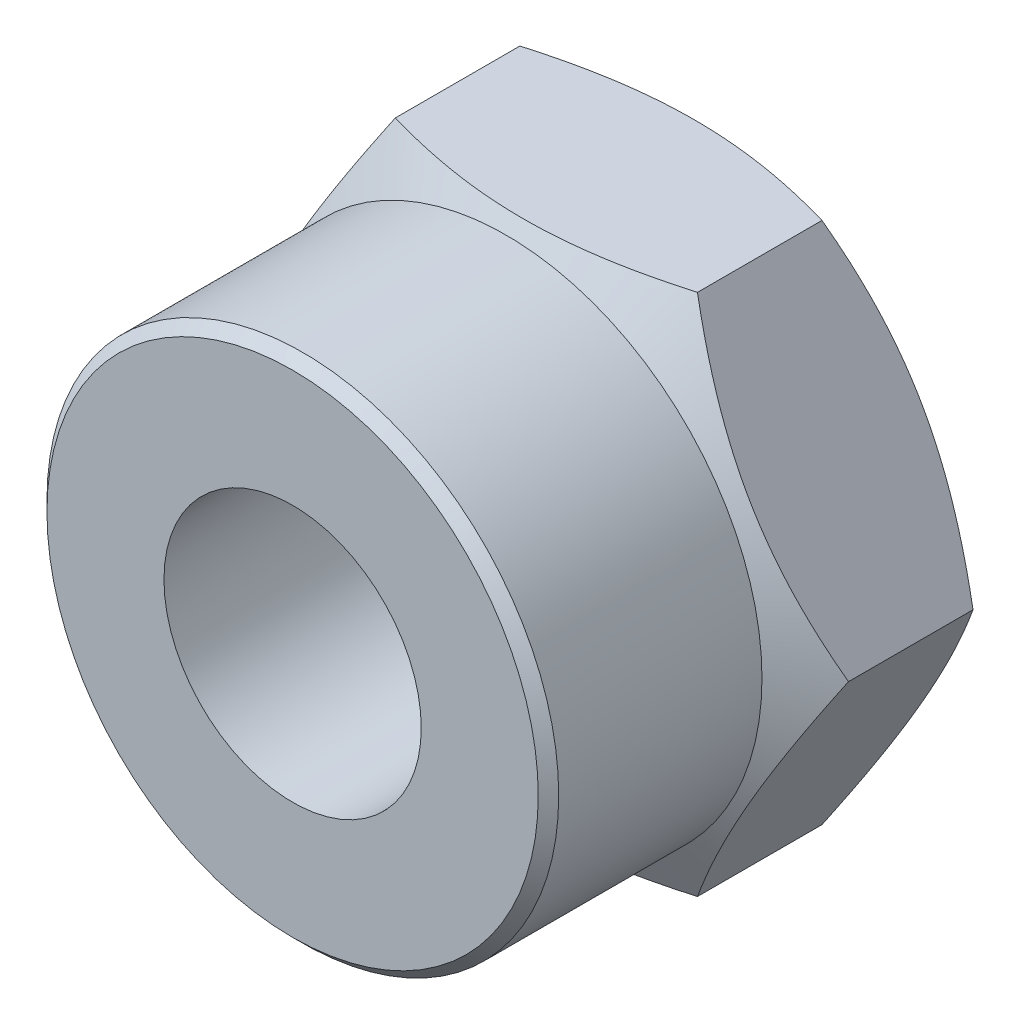
SolidWorks part; units mm, degrees
ref_plane "Front" through (0, 0, 0) normal (0, 0, 1) x (1, 0, 0)
ref_plane "Top" through (0, 0, 0) normal (0, 1, 0) x (1, 0, 0)
ref_plane "Right" through (0, 0, 0) normal (1, 0, 0) x (0, 0, -1)
sketch "Sketch1" plane through (0, 0, 0) normal (0, 0, 1) x (1, 0, 0)
  line L1 (2.8868, -5) -> (5.7735, 0)
  line L2 (5.7735, 0) -> (2.8868, 5)
  line L3 (2.8868, 5) -> (-2.8868, 5)
  line L4 (-2.8868, 5) -> (-5.7735, 0)
  line L5 (-5.7735, 0) -> (-2.8868, -5)
  line L6 (-2.8868, -5) -> (2.8868, -5)
  circle A0 centre (0, 0) radius 5 construction
  circle A1 centre (0, 0) radius 2.4585
extrude "BaseNut" add sketch "Sketch1" against normal blind 3.92
cosmetic thread "ThreadCosmetic1" [suppressed] parameters "m"=4.9, "D2"=6
sketch "Sketch3" plane through (0, 0, 0) normal (0, 1, 0) x (1, 0, 0)
  line L0 (0, 16.3108) -> (0, -16.1137) construction
  line L2 (-2.0696, 1.96) -> (33.5085, 1.96) construction
  line L3 (4.44, 3.92) -> (5.7735, 3.92)
  line L5 (5.7735, 3.92) -> (5.7735, 3.1501)
  line L7 (5.7735, 3.1501) -> (4.44, 3.92)
  line L8 (5.7735, 0.7699) -> (4.44, 0)
  line L9 (5.7735, 0) -> (5.7735, 0.7699)
  line L10 (4.44, 0) -> (5.7735, 0)
  dimension "D1" = 30
  dimension "dw" = 8.88
revolve "Double-Chamfer" cut sketch "Sketch3" angle 360 about L0
sketch "Sketch2" plane through (20.0871, -4.2815, 0) normal (0, 0, 1) x (1, 0, 0)
  circle A1 centre (-20.0871, 4.2815) radius 2.4585 construction
  circle A2 centre (-20.0871, 4.2815) radius 4.89
  circle A3 centre (-20.0871, 4.2815) radius 2.4585
extrude "Extrude1" add sketch "Sketch2" along normal offset from surface (4.08 mm away) 8 up to face at (2.4585, 0, -3.92)
sketch "Sketch5" plane through (0, 0, 0) normal (0, 1, 0) x (1, 0, 0)
  line L0 (0, 16.8008) -> (0, -2.8116) construction
  line L2 (2.4585, 3.92) -> (3.375, 3.92)
  line L5 (3.375, 3.92) -> (2.4585, 3.0035)
  line L7 (2.4585, 3.0035) -> (2.4585, 3.92)
  dimension "D1" = 45
  dimension "da" = 6.75
revolve "EndChamfer" cut sketch "Sketch5" angle 360 about L0
chamfer "Chamfer1" distance 0.1956 angle 45 1 edges at (4.89, 0, 4.08)
sketch "Sketch6" plane through (0, 0, 0) normal (0, 1, 0) x (1, 0, 0)
  line L0 (0, 30.0005) -> (0, -32.7386) construction
  line L1 (1.917, 3.2743) -> (2.4585, 3.2743)
  line L2 (2.4585, 3.2743) -> (2.9275, 3.0035)
  line L3 (2.9275, 3.0035) -> (2.4585, 2.7328)
  line L4 (2.4585, 2.7328) -> (1.917, 2.7328)
  line L5 (1.917, 2.7328) -> (1.917, 3.2743)
  line L6 (-2.4585, 3.0035) -> (2.4585, 3.0035) construction
revolve "Cut-Revolve10" [suppressed] cut sketch "Sketch6" angle 360 about L0
pattern_linear "LPattern10" [suppressed] count 6 spacing 0.6498 along (0, 0, 1)
equation "\"D1@Chamfer1\" = \"s1@Sketch2\" / 50"
equation "\"D2@Sketch6\" = \"xd@Sketch1\""
equation "\"D1@Sketch6\" = (  \"D2@ThreadCosmetic1\" - \"xd@Sketch1\" )  / 2"
equation "\"D3@LPattern10\" = \"D1@Sketch6\" * 1.2"
equation "\"D1@LPattern10\" = \"m1@BaseNut\" / \"D3@LPattern10\""
